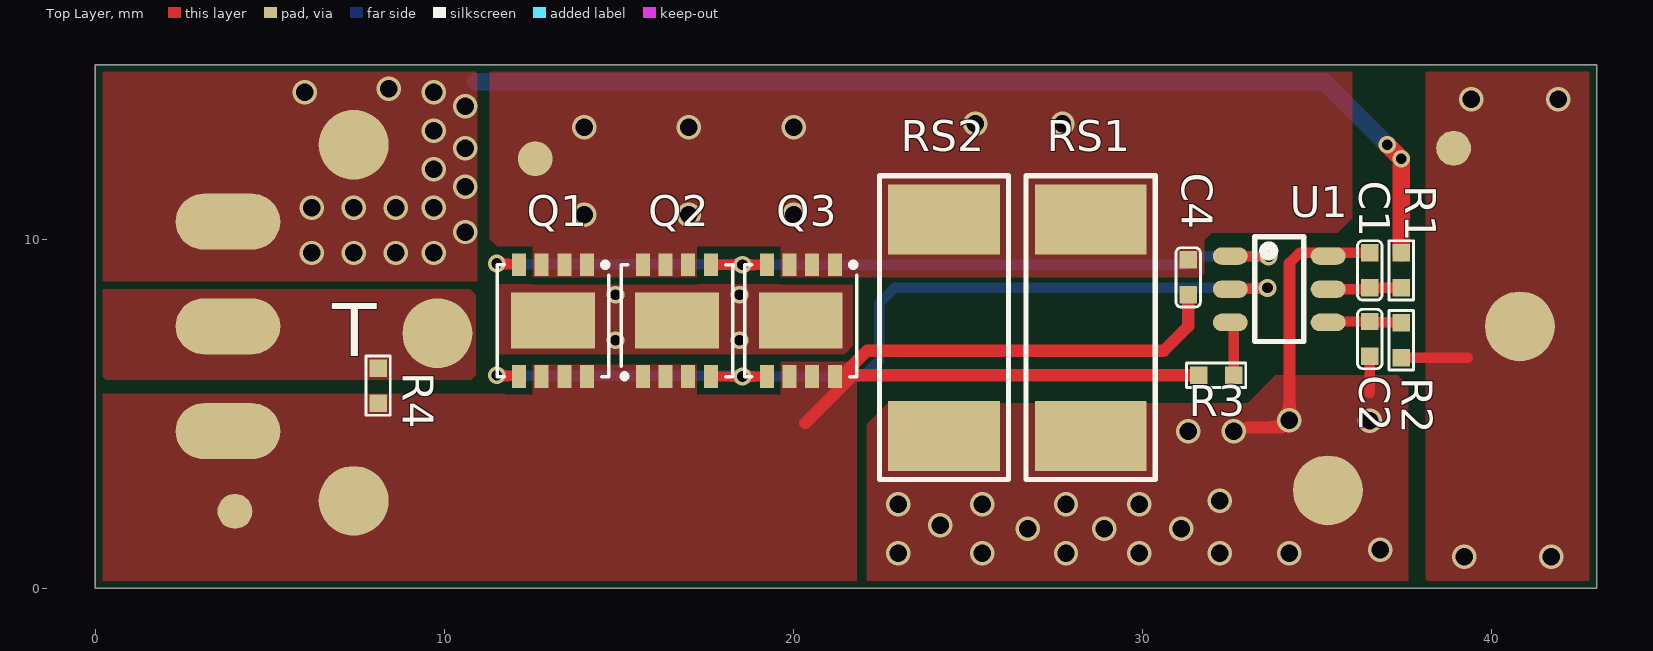
[diagram p0: Top Layer view]
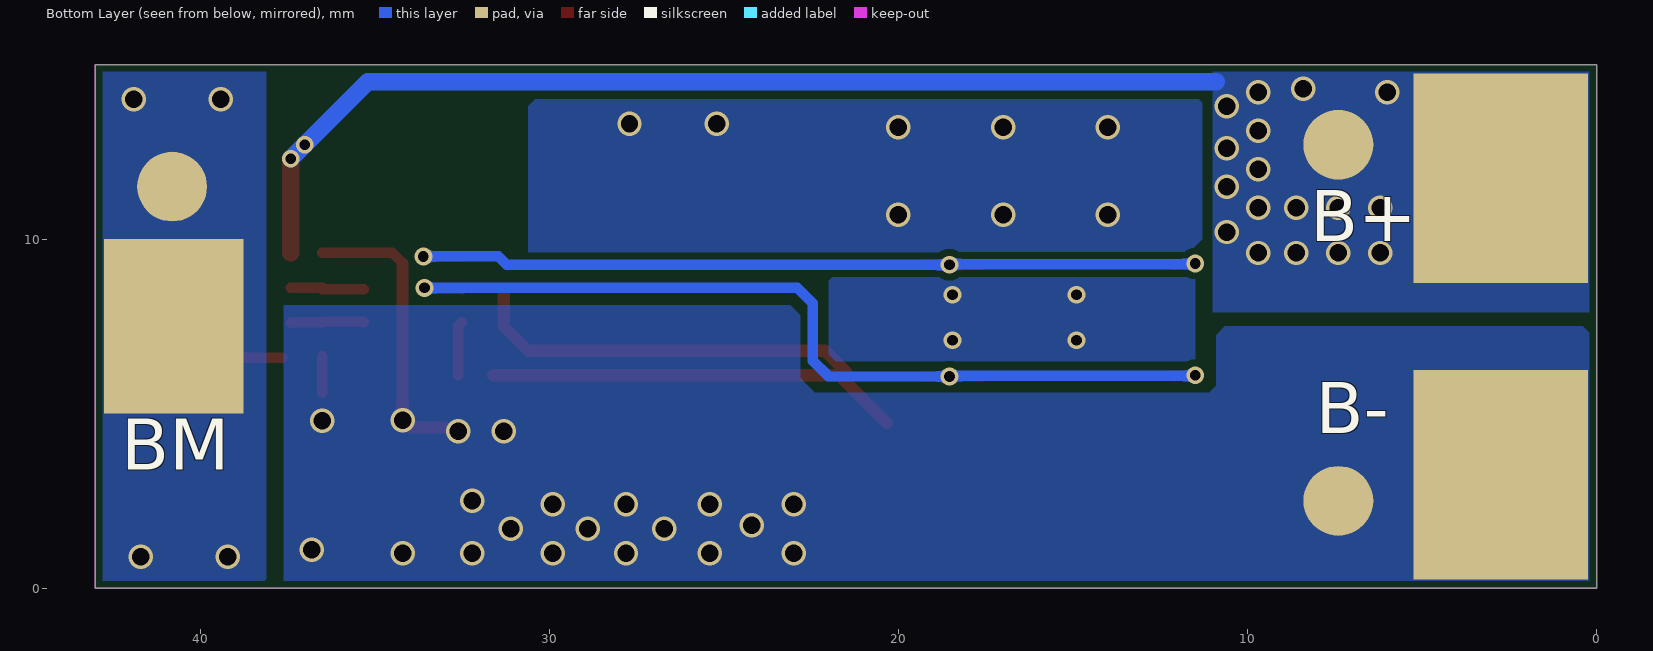
[diagram p1: Bottom Layer view, seen from below]
# Altium PCB MISC78884.PcbDoc
Units mm, origin at the board's own origin, x right, y up, seen from the top; angles counter-clockwise.
Board outline 43 x 15 mm, 2 copper layers (Top Layer, Bottom Layer); 17 components, 12 nets, 68 pads, 61 vias.

## Layer stack, top to bottom (the 12.6 mil dielectric is the usual default, probably not edited)
Top Solder: solder mask 0.0102, Solder Resist, Dk 3.5
Top Layer: signal copper 0.0356
Dielectric 1: dielectric 0.32, FR-4, Dk 4.8
Bottom Layer: signal copper 0.0356
Bottom Solder: solder mask 0.0102, Solder Resist, Dk 3.5

## Board outline
0,-0.003 43,-0.003 43,14.997 0,14.997

## Design rules (kind name [scope] priority, off if disabled: settings)
Clearance [All] p1: gap=0.2 ignorepadtopadclearanceinfootprint=TRUE
MinimumSolderMaskSliver [All] p1: minsoldermaskwidth=0.01
PolygonConnect [All] p1: connectstyle=Direct reliefconductorwidth=0.254 reliefentries=4 polygonreliefangle="90 Angle" airgapwidth=0.254
RoutingVias [All] p1: holewidth=0.711 width=1.27 viastyle="Through Hole" minholewidth=0.711 minwidth=1.27 maxholewidth=0.711 maxwidth=1.27
SilkToSilkClearance [All] p1: silktosilkclearance=0
SilkToSolderMaskClearance [IsPad] p1: minsilkscreentomaskgap=0 clearancetoexposedcopper=TRUE
SolderMaskExpansion [All] p1: expansion=0.102 istentingtop=FALSE
Width [All] p1: maxlimit=10 minlimit=0.254 preferedwidth=0.254
27 further rules are at their usual default settings.

## Components (designator, comment, footprint, x,y, rotation, side; value= is the part's Value field where it differs from the comment)
B+ "Pad" Pad10X8mm#1 2.75,11.747 r90 bottom locked
B- "Pad" Pad10X8mm#1 2.75,3.247 r270 bottom locked
BM "Pad" Pad10X8mm#2 40.75,7.497 r90 bottom locked
C1 "0.1uF" C0402A 36.5,9.1 r270 top
C2 "0.1uF" C0402A 36.5,7.137 r90 top
C4 "0.1uF" C0402A 31.3,8.9 r90 top
Q1 "N MOS" DFN3*3-L8(2N) 13.107,7.662 r180 top
Q2 "N MOS" DFN3*3-L8(2N) 16.657,7.662 r0 top
Q3 "N MOS" DFN3*3-L8(2N) 20.207,7.662 r180 top
R1 "470R" R0402A 37.4,9.1 r270 top
R2 "470R" R0402A 37.4,7.1 r90 top
R3 "2K" R0402A 32.1,6.1 r0 top
R4 "10K" R0402A 8.1,5.8 r90 top
RS1 "R010" R2512L 28.507,7.462 r90 top
RS2 "R010" R2512L 24.307,7.462 r90 top
T "Pad" Pad10X8mm#3 3.8,7.497 r270 top locked
U1 "CM1020*" SOT23-6A 33.907,8.562 r0 top

## Footprints (in the part's own frame and the unit in brackets; to place one, negate y for a bottom-side part, rotate by r counter-clockwise, add the part's x,y. Pads: shape width x height; smd on the part's side, far side on the other; paste and mask are expansions set on the pad)
C0402A [mm] "贴片电容"
  rect 0.5x0.5 smd paste+0 mask+0.05: 1(-0.5,0) 2(0.5,0)
  silkscreen extent -0.85,-0.35 0.85,0.35
DFN3*3-L8(2N) [mm] "DFN3*3双管贴片MOS"
  rect 0.4x0.65 smd: 1(-0.975,-1.6) 2(-0.325,-1.6) 3(0.325,-1.6) 4(0.975,-1.6) 5(0.975,1.6) 6(0.325,1.6) 7(-0.325,1.6) 8(-0.975,1.6)
  rect 2.4x1.6 smd: 9(0,0)
  silkscreen extent -1.6,-1.6 1.6,1.6
Pad10X8mm#1 [mm]
  rect 6x5 smd: 1(0,0)
Pad10X8mm#2 [mm]
  rect 5x4 smd: 1(0,0)
Pad10X8mm#3 [mm]
  oval 1.6x3 smd: 1(0,0)
R0402A [mm] "贴片电阻"
  rect 0.5x0.5 smd paste+0 mask+0.05: 1(-0.5,0) 2(0.5,0)
  silkscreen extent -0.85,-0.35 0.85,0.35
R2512L [mm] "贴片电阻"
  rect 2x3.2 smd: 1(-3.1,0) 2(3.1,0)
  silkscreen extent -4.35,-1.85 4.35,1.85
SOT23-6A [mm]
  oval 1x0.5 smd mask+0.05: 1(-1.4,0.95) 2(-1.4,0) 3(-1.4,-0.95) 4(1.4,-0.95) 5(1.4,0) 6(1.4,0.95)
  silkscreen extent -0.7,-1.5 0.7,1.5

## Part data
B+ B- BM T: "Connection pad (non-through-hole)"
C1 C2 C4: library part CAP, "SMD capacitor"
Q1 Q2 Q3: library part "2N MOS", "SMD MOS-TSSOP-8"
R1 R2 R3 R4: library part RES, "SMD resistor"
RS1 RS2: library part RES2, "SMD alloy resistor"
U1: library part S-8252, "2S battery protection IC"

## Free pads (board coordinates)
  round 2 smd: 2(7.4,2.5) 2(7.4,12.7) 2(9.8,7.3) 2(35.3,2.8) 2(40.8,7.497)
  round 2 smd far side: 2(7.4,2.5) 2(7.4,12.7) 2(40.8,11.5)
  round 1 smd: 3(4,2.2) 3(12.6,12.3) 3(38.9,12.6)
  oval 3x1.6 smd: 4(3.8,4.497) 4(3.8,10.497)

## Via types
v1: diameter 0.7, hole 0.5, Top Layer to Bottom Layer, tented both sides, 49 vias
v2: diameter 0.508, hole 0.305, Top Layer to Bottom Layer, tented both sides, 12 vias

## Nets (pads, with @x,y where several pads share a name; then routed paths per layer and width w, separated by ;. In a path a pad name is that pad's centre, name@x,y a point inside that pad or via, vN(x,y) a via of type N, cw(c..) or ccw(c..) an arc to the next point about the centre after c; other vN are vias at no path point)
B+: B+.1 pad.2@7.4,12.7 pad.4@3.8,10.497 R1.1 | length 30.7
  Top Layer w0.5: v2(37,12.7) 37,12.698 37.4,12.298 R1.1
  Bottom Layer w0.5: 10.9,14.5 35.2,14.5 v2(37,12.7) v2(37.4,12.3)
  other v1: 6.2,9.6 7.4,9.6 8.6,9.6 9.7,9.6 10.6,10.2 6.2,10.9 7.4,10.9 8.6,10.9 9.7,10.9 10.6,11.5 9.7,12 10.6,12.6 9.7,13.1 10.6,13.8 6,14.2 9.7,14.2 8.4,14.3
B-: B-.1 C1.1 C2.1 pad.2@7.4,2.5 pad.2@35.3,2.8 RS1.1 RS2.1 U1.6 | length 9.2
  Top Layer w0.3: 34.2,9.3 34.5,9.6 C1.1 ; 36.5,5.6 C2.1
  Top Layer w0.35: 33,4.6 33.995,4.6 v1(34.2,4.805) 34.2,9.3
  other v1: 23,1 25.4,1 27.8,1 29.9,1 32.2,1 34.2,1 36.8,1.1 26.7,1.7 28.9,1.7 31.1,1.7 24.2,1.8 23,2.4 25.4,2.4 27.8,2.4 29.9,2.4 32.2,2.5 31.3,4.5 32.6,4.5 36.5,4.8
BM: BM.1 pad.2@40.8,7.497 pad.2@40.8,11.5 pad.3@38.9,12.6 R2.1 | length 1.7
  Top Layer w0.3: R2.1@37.64,6.6 39.304,6.6
  other v1: 39.2,0.9 41.7,0.9 39.4,14 41.9,14
CO: Q1.5 Q2.4 Q3.5 U1.2 | length 27.4
  Top Layer w0.3: v2(11.5,6.1) 11.519,6.081 12.113,6.081 Q1.5 ; Q2.4 v2(18.538,6.062) Q3.5 ; U1.2 32.526,8.581 33.552,8.581 v2(33.571,8.6)
  Bottom Layer w0.3: v2(11.5,6.1) 11.519,6.081 18.519,6.081 v2(18.538,6.062) 22,6.062 22.457,6.519 22.457,8.157 22.9,8.6 v2(33.571,8.6)
D: Q1.9 Q2.9 Q3.9
  other v2: 14.9,7.1 18.45,7.1 14.9,8.4 18.45,8.4
DO: Q1.4 Q2.5 Q3.4 U1.1 | length 25.6
  Top Layer w0.3: v2(11.5,9.3) 11.519,9.281 12.113,9.281 Q1.4 ; Q2.5 v2(18.538,9.262) Q3.4 ; U1.1 32.514,9.505 33.595,9.505 v2(33.603,9.497)
  Bottom Layer w0.3: v2(11.5,9.3) 11.519,9.281 18.519,9.281 v2(18.538,9.262) 31.22,9.262 31.458,9.5 33.6,9.5 v2(33.603,9.497)
NetC1_2: C1.2 R1.2 U1.5 | length 2.1
  Top Layer w0.3: U1.5 C1.2@36.5,8.562 ; C1.2 R1.2
NetC2_2: C2.2 R2.2 U1.4 | length 2.1
  Top Layer w0.3: U1.4 35.332,7.637 C2.2 36.519,7.619 37.381,7.619 R2.2
NetC4_2: C4.2 pad.3@12.6,12.3 Q1.1 Q1.2 Q1.3 Q2.6 Q2.7 Q2.8 Q3.1 Q3.2 Q3.3 RS1.2 RS2.2
  other v1: 14,10.7 17,10.7 20,10.7 14,13.2 17,13.2 20,13.2 25.2,13.3 27.7,13.3
NetR3_2: R3.2 U1.3 | length 1.6
  Top Layer w0.3: U1.3@32.508,7.612 32.6,7.52 R3.2
P-: C4.1 pad.2@7.4,2.5 pad.3@4,2.2 pad.4@3.8,4.497 Q1.6 Q1.7 Q1.8 Q2.1 Q2.2 Q2.3 Q3.6 Q3.7 Q3.8 R3.1 R4.1 | length 23.1
  Top Layer w0.35: 20.331,4.731 21.7,6.1 R3.1 ; 21.5,6.2 22.1,6.8 30.6,6.8 31.3,7.5 C4.1
T: pad.2@9.8,7.3 R4.2 T.1

## Polygon pours and split planes (outlines as drawn)
B- on Bottom Layer "NONET_L02_P-001" (solid, remove dead copper, pour order 1): 22.814,7.814 23.1,8.1 37.6,8.1 37.6,0 0,0 0.107,0.107 0.107,7.212 0.395,7.5 10.65,7.5 10.9,7.25 10.9,5.8 11.1,5.6 22.4,5.6 22.814,6.014
D on Bottom Layer "NONET_L02_P-001" (solid, remove dead copper, pour order 11): 11.5,8.9 11.5,6.5 21.8,6.5 22,6.7 22,8.8 21.9,8.9
NetC4_2 on Bottom Layer "NONET_L02_P-001" (solid, remove dead copper, pour order 8): 30.6,9.619 11.681,9.619 11.3,10 11.3,13.9 11.4,14 30.4,14 30.6,13.8 30.6,11.284
B+ on Bottom Layer "NONET_L02_P-001" (solid, remove dead copper, pour order 2): 0.107,14.962 0.207,15.062 11,15.062 11,7.9 0.107,7.9
BM on Bottom Layer "NONET_L02_P-001" (solid, remove dead copper, pour order 0): 38.107,15.062 38.107,0.262 38.369,0 43,0 43,14.994
D on Top Layer "NONET_L02_P-001" (solid, remove dead copper, pour order 10): 21.7,6.941 21.459,6.7 11.5,6.7 11.5,8.7 21.7,8.7
B- on Top Layer "NONET_L02_P-001" (solid, remove dead copper, pour order 5): 33,5.3 33.8,6.1 37.3,6.1 37.6,5.8 37.6,0.162 22.1,0.162 22.1,4.7 22.7,5.3 26.25,5.3
B+ on Top Layer "NONET_L02_P-001" (solid, remove dead copper, pour order 6): 0,14.997 0,8.997 0.2,8.797 10.941,8.797 10.941,14.728 10.807,14.862 -0.093,14.862 -0.493,15.262
BM on Top Layer "NONET_L02_P-001" (solid, remove dead copper, pour order 9): 38.107,15.062 38.107,0.262 38.372,-0.003 42.997,-0.003 42.997,14.99 43,14.994
T on Top Layer "NONET_L02_P-001" (solid, remove dead copper, pour order 7): 10.762,5.962 10.9,6.1 10.9,8.4 10.738,8.562 0.207,8.562 0.207,6.062 0.307,5.962
P- on Top Layer "NONET_L02_P-001" (solid, remove dead copper, pour order 4): 17.232,6.4 17.232,5.537 19.632,5.537 19.632,6.487 21.807,6.487 21.807,-0.038 0.407,-0.038 -0.093,0.462 0.107,0.662 0.107,5.562 12.457,5.562 12.507,5.612 12.507,6.4
NetC4_2 on Top Layer "NONET_L02_P-001" (solid, remove dead copper, pour order 3): 35.581,10.181 36,10.6 36,14.8 35.738,15.062 11.462,15.062 11.3,14.9 11.3,10 11.513,9.787 12.532,9.787 12.532,8.987 12.507,8.962 12.538,8.9 17.232,8.9 17.232,9.787 19.632,9.787 19.632,8.9 31.65,8.9 31.761,9.011 31.761,9.961 31.981,10.181

## Keep-outs
Keep-Out Layer:
  the board outline again, w0.013

## Silkscreen, mask and mechanical layers (free items; w line width, h text height)
Mechanical 1:
  the board outline again, w0.006